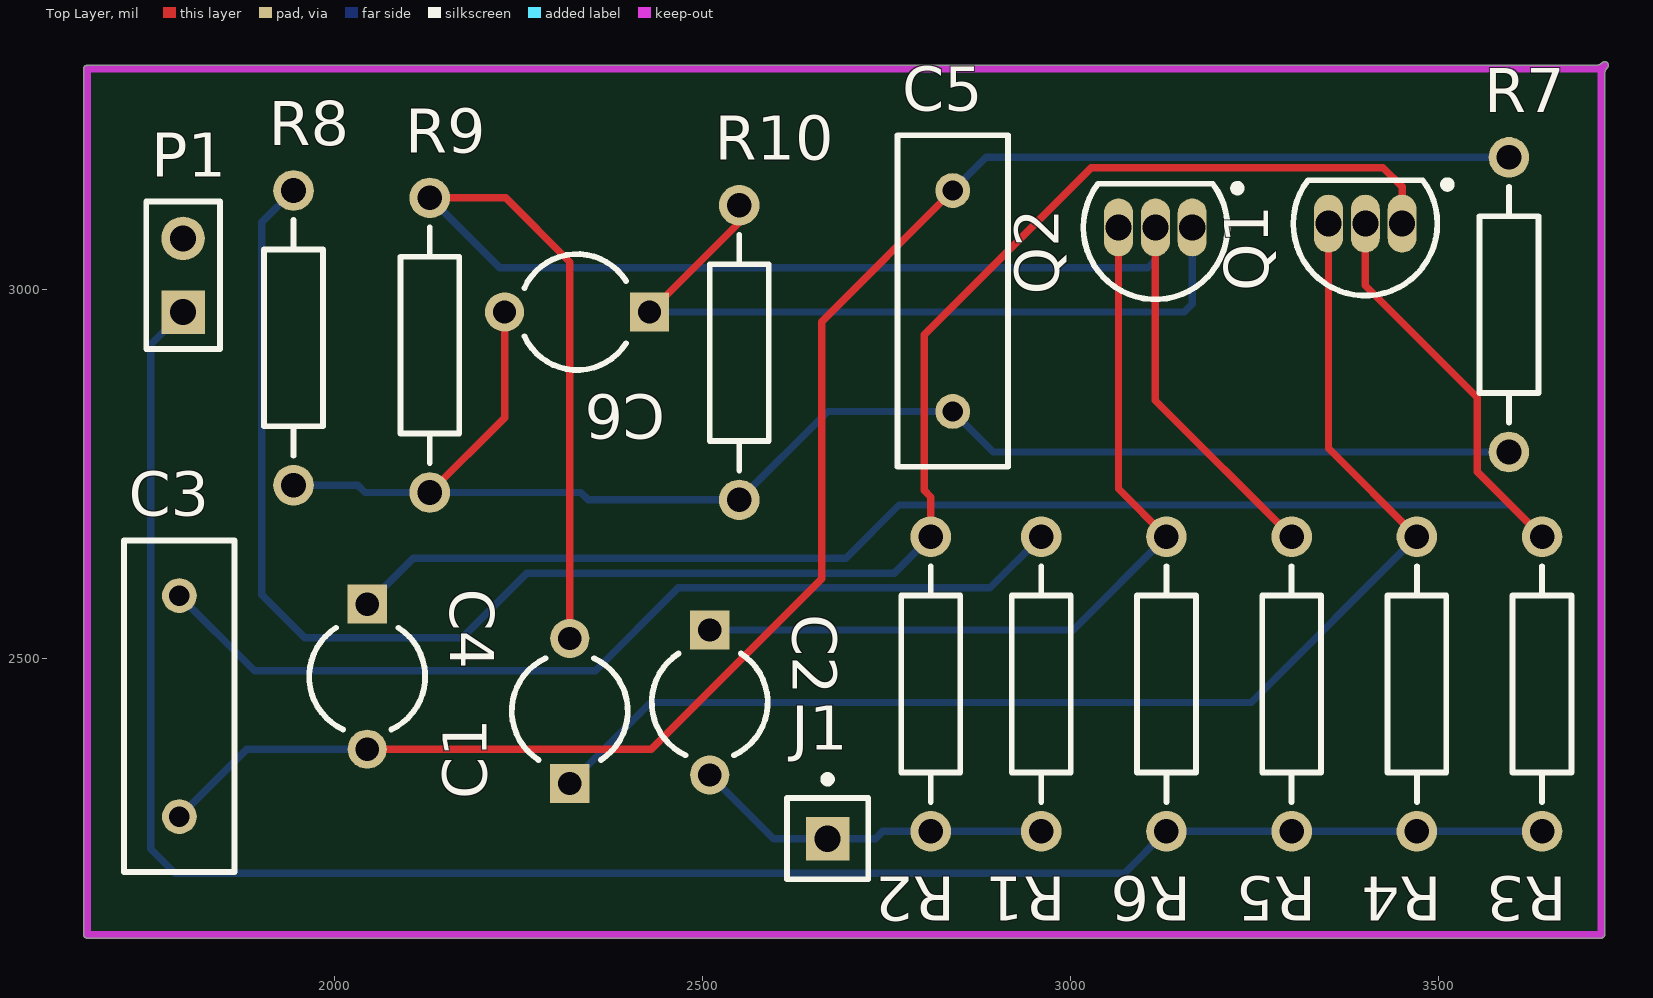
[diagram p0: Top Layer view]
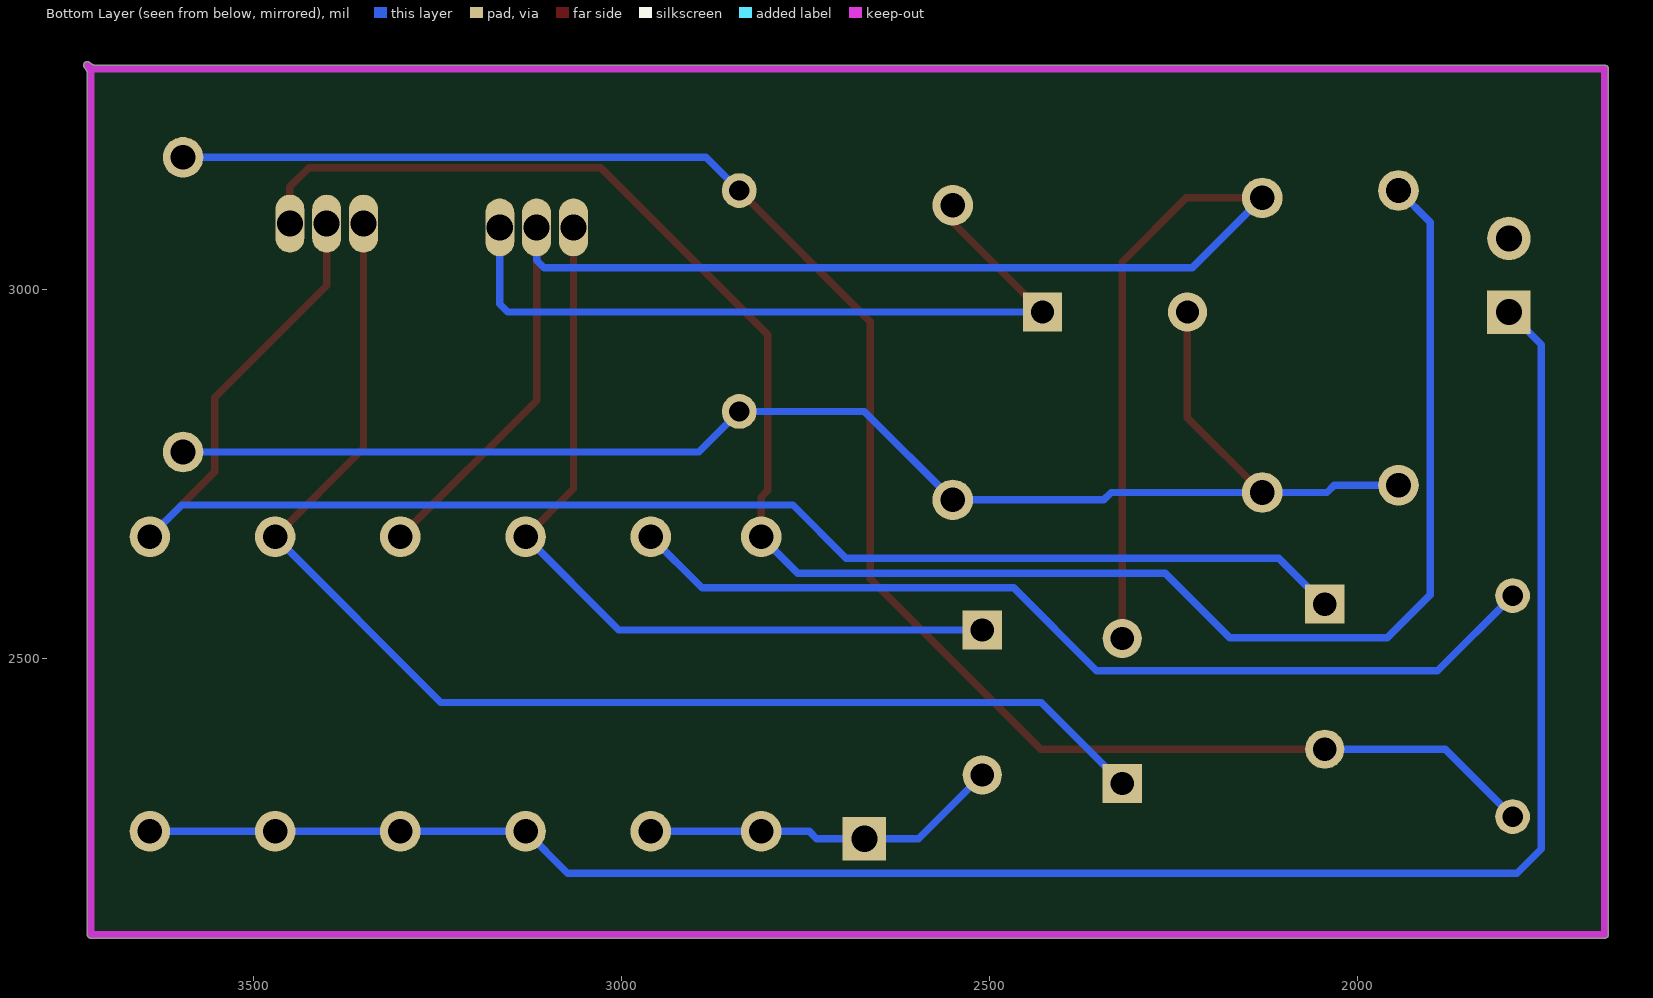
[diagram p1: Bottom Layer view, seen from below]
# Altium PCB MISC82905.PcbDoc
Units mil, origin at the board's own origin, x right, y up, seen from the top; angles counter-clockwise.
Board outline 2070.03 x 1190.02 mil, 2 copper layers (Top Layer, Bottom Layer); 20 components, 12 nets, 41 pads, 0 vias.

## Layer stack, top to bottom (the 12.6 mil dielectric is the usual default, probably not edited)
Top Solder: solder mask 0.4, Solder Resist, Dk 3.5
Top Layer: signal copper 1.4
Dielectric 1: dielectric 12.6, FR-4, Dk 4.8
Bottom Layer: signal copper 1.4
Bottom Solder: solder mask 0.4, Solder Resist, Dk 3.5

## Board outline
1659.98,2125 1659.98,3300 cw(c1665,3300) 1665,3305.01 3712.93,3305.01 ccw(c3712.93,3317.07) 3721.45,3308.55 cw(c3725,3305) 3730.01,3305 cw(c3725,3305) 3728.55,3301.45 ccw(c3737.07,3292.93) 3725.01,3292.93 cw(c3720,3292.93) 3725.01,3292.93 cw(c3720,3292.93) 3725.01,3292.93 3725.01,2125 cw(c3720,2125) 3720,2119.99 1665,2119.99 cw(c1665,2125)

## Design rules (kind name [scope] priority, off if disabled: settings)
Clearance [All] p1: gap=10
PolygonConnect [All] p1: connectstyle=Relief reliefconductorwidth=10 reliefentries=4 polygonreliefangle="90 Angle" airgapwidth=10
RoutingVias [All] p1: holewidth=28 width=50 viastyle="Through Hole" minholewidth=28 minwidth=50 maxholewidth=28 maxwidth=50
SolderMaskExpansion [All] p1: expansion=4
Width [All] p1: maxlimit=10 minlimit=10 preferedwidth=10
30 further rules are at their usual default settings.

## Components (designator, comment, footprint, x,y, rotation, side; value= is the part's Value field where it differs from the comment)
C1 "10uF" CAPR5-4X5 2320,2428.43 r90 top
C2 "10uF" CAPR5-4X5 2510,2440 r270 top
C3 "0.01uF" RAD-0.3 1790,2435 r90 top
C4 "10uF" CAPR5-4X5 2045,2475 r270 top
C5 "0.01uF" RAD-0.3 2840,2985 r90 top
C6 "10uF" CAPR5-4X5 2330,2970 r180 top
J1 "Socket" PIN1 2670,2255 r0 top
P1 "Header 2" HDR1X2 1795,2970 r90 top
Q1 "9013" TO-92A 3400,3090 r90 top
Q2 "9013" TO-92A 3115,3085 r90 top
R1 "16K" AXIAL-0.4 2960,2465 r270 top
R2 "10K" AXIAL-0.4 2810,2465 r270 top
R3 "10K" AXIAL-0.4 3640,2465 r270 top
R4 "10K" AXIAL-0.4 3470,2465 r270 top
R5 "10K" AXIAL-0.4 3300,2465 r270 top
R6 "5.1K" AXIAL-0.4 3130,2465 r270 top
R7 "16K" AXIAL-0.4 3595,2980 r90 top
R8 "1.2K" AXIAL-0.4 1945,2935 r90 top
R9 "10K" AXIAL-0.4 2130,2925 r90 top
R10 "470" AXIAL-0.4 2550,2915 r90 top

## Footprints (in the part's own frame and the unit in brackets; to place one, negate y for a bottom-side part, rotate by r counter-clockwise, add the part's x,y. Pads: shape width x height; smd on the part's side, far side on the other; paste and mask are expansions set on the pad)
AXIAL-0.4 [mm] "Axial Device, Thru-Hole; 2 Leads; 0.4 in Pin Spacing"
  round 1.4 hole 0.85: 1(-5.08,0) 2(5.08,0)
  silkscreen extent -4.06,-1.02 4.06,1.02
CAPR5-4X5 [mm] "Capacitor; 2 Leads"
  rect 1.35x1.35 hole 0.8: 1(-2.5,0)
  round 1.35 hole 0.8: 2(2.5,0)
  silkscreen extent -1.69,-2 1.82,2
HDR1X2 [mm] "Connector; Header; 2 Position"
  rect 1.5x1.5 hole 0.9: 1(0,0)
  round 1.5 hole 0.9: 2(2.54,0)
  silkscreen extent -1.27,-1.27 3.81,1.27
PIN1 [mm] "Connector; Plug"
  rect 1.5x1.5 hole 0.9: 1(0,0)
  silkscreen extent -1.4,-1.4 1.4,2.17
RAD-0.3 [mm] "Radial Cap, Thru-Hole; 2 Leads; 0.3 in Pin Spacing"
  round 1.2 hole 0.7: 1(-3.81,0) 2(3.81,0)
  silkscreen extent -5.71,-1.91 5.71,1.91
TO-92A [mm] "TO, Flat Index; 3 In-Line, Axial Leads; Body Dia. 4.5mm; Leads 0.51 x 0.48 mm (max)"
  oval 2x1 hole 0.9: 1(0,-1.27) 2(0,0) 3(0,1.27)
  silkscreen extent -2.48,-2.96 1.5,2.48, body extent -2.48,-2.5 1.5,2.5, height 6.86

## Part data
C1 C2 C4 C6: library part Cap2, "Capacitor"
C3 C5: library part Cap, "Capacitor"
P1: "Header, 2-Pin"
Q1 Q2: library part 2N3904, "NPN General Purpose Amplifier"
R1 R2 R3 R4 R5 R6 R7 R8 R9 R10: library part Res2, "Resistor"

## Nets (pads, with @x,y where several pads share a name; then routed paths per layer and width w, separated by ;. In a path a pad name is that pad's centre, name@x,y a point inside that pad or via, vN(x,y) a via of type N, cw(c..) or ccw(c..) an arc to the next point about the centre after c; other vN are vias at no path point)
+12V: P1.1 R3.2 R4.2 R5.2 R6.2 | length 2673.5
  Bottom Layer w10: P1.1 1751,2926 1751,2241 1784,2208 3073,2208 R6.2 R5.2 R4.2 R3.2
GND: P1.2
NetC1_1: C1.1 Q1.3 R4.1 | length 1763.5
  Top Layer w10: Q1.3 3350,2785 R4.1
  Bottom Layer w10: C1.1 2430,2440 3245,2440 R4.1
NetC1_2: C1.2 Q2.2 R5.1 R9.2 | length 2307.3
  Top Layer w10: R9.2 2233,3125 2320,3038 C1.2 ; Q2.2 3115,2850 R5.1
  Bottom Layer w10: R9.2 2225,3030 3105,3030 3115,3040 Q2.2
NetC2_1: C2.1 Q2.3 R6.1 | length 1119.4
  Top Layer w10: Q2.3 3065,2730 R6.1
  Bottom Layer w10: C2.1 3003.43,2538.43 R6.1
NetC2_2: C2.2 J1.1 R1.2 R2.2 | length 490
  Bottom Layer w10: C2.2 2596.57,2255 J1.1 2735,2255 2745,2265 R2.2 R1.2
NetC3_1: C3.1 C4.2 C5.2 R7.2 | length 2380.2
  Top Layer w10: C4.2 2430.57,2376.57 2662,2608 2662,2957 C5.2
  Bottom Layer w10: C3.1 1881.57,2376.57 C4.2 ; C5.2 2885,3180 R7.2
NetC3_2: C3.2 R1.1 | length 1287.6
  Bottom Layer w10: C3.2 1892,2483 2355,2483 2467.49,2595.49 2890.49,2595.49 R1.1
NetC4_1: C4.1 Q1.2 R3.1 | length 2193
  Top Layer w10: Q1.2 3400,3006 3552,2854 3552,2753 R3.1
  Bottom Layer w10: C4.1 2107.57,2636 2695,2636 2767,2708 3597,2708 R3.1
NetC5_1: C5.1 C6.2 R7.1 R8.1 R9.1 R10.1 | length 2017.8
  Top Layer w10: R9.1 2231.57,2826.57 C6.2
  Bottom Layer w10: R8.1 2032,2735 2042,2725 R9.1 2335,2725 2345,2715 R10.1 2670,2835 C5.1 2895,2780 R7.1
NetC6_1: C6.1 Q2.1 R10.2 | length 1040.5
  Top Layer w10: C6.1 2550,3091.57 R10.2
  Bottom Layer w10: C6.1 3154,2970 3165,2981 Q2.1
NetQ1_1: Q1.1 R2.1 R8.2 | length 2637.1
  Top Layer w10: R2.1 2810,2719 2801,2728 2801,2939 3028,3166 3424,3166 3450,3140 Q1.1
  Bottom Layer w10: R8.2 1902,3092 1902,2586 1960,2528 2174,2528 2261.5,2615.5 2760.5,2615.5 R2.1

## Keep-outs
Keep-Out Layer:
  lines w10: 1665,2125 1665,3300 3712.93,3300 ccw(c3712.93,3317.07) 3725,3305 ccw(c3737.07,3292.93) 3720,3292.93 3720,2125 1665,2125